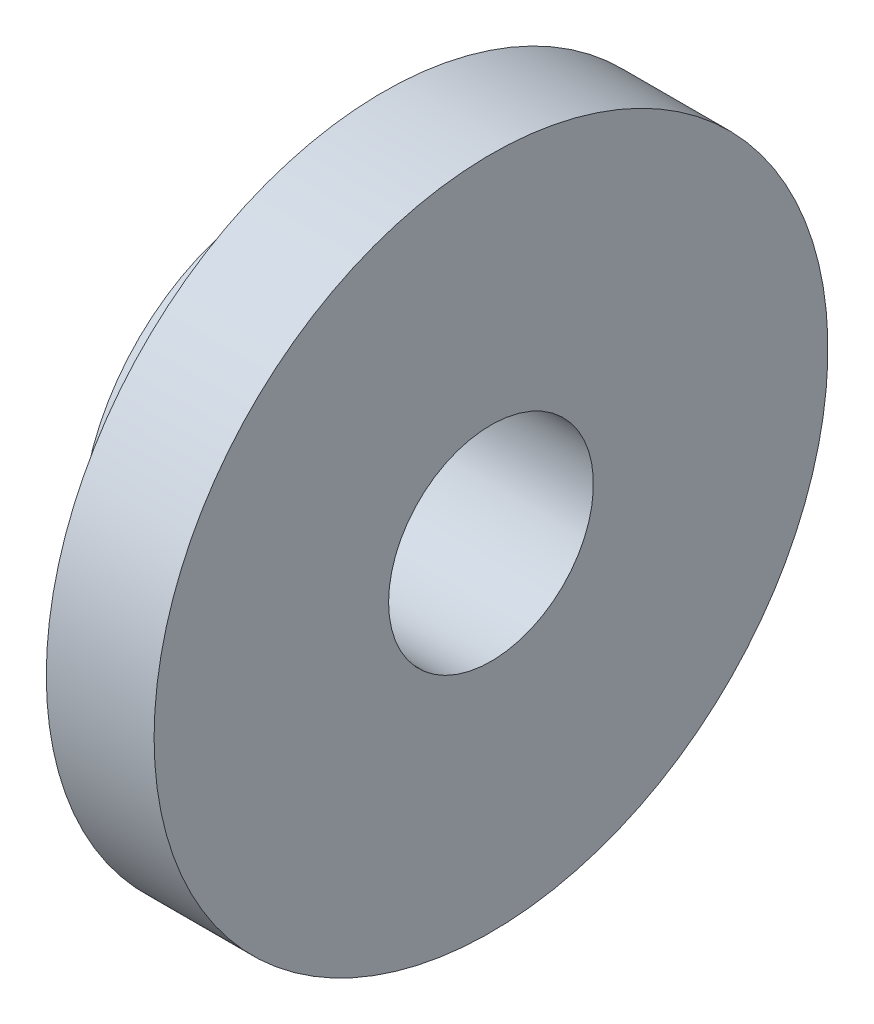
SolidWorks part; units mm, degrees
material "35"
ref_plane "Front Plane" through (0, 0, 0) normal (0, 0, 1) x (1, 0, 0)
ref_plane "Top Plane" through (0, 0, 0) normal (0, 1, 0) x (1, 0, 0)
ref_plane "Right Plane" through (0, 0, 0) normal (1, 0, 0) x (0, 0, -1)
sketch "Sketch1" plane through (0, 0, 0) normal (0, 0, 1) x (1, 0, 0)
  line L0 (0, 0) -> (78.9231, 0) construction
  line L1 (0, -19) -> (0, -36)
  line L2 (0, -36) -> (20, -36)
  line L3 (20, -36) -> (20, -62.5)
  line L4 (20, -62.5) -> (40, -62.5)
  line L5 (40, -62.5) -> (40, -19)
  line L6 (40, -19) -> (0, -19)
  dimension "D1" = 19
  dimension "D2" = 36
  dimension "D3" = 62.5
  dimension "D4" = 40
  dimension "D5" = 20
revolve "Revolve1" add sketch "Sketch1" angle 360 about L0
